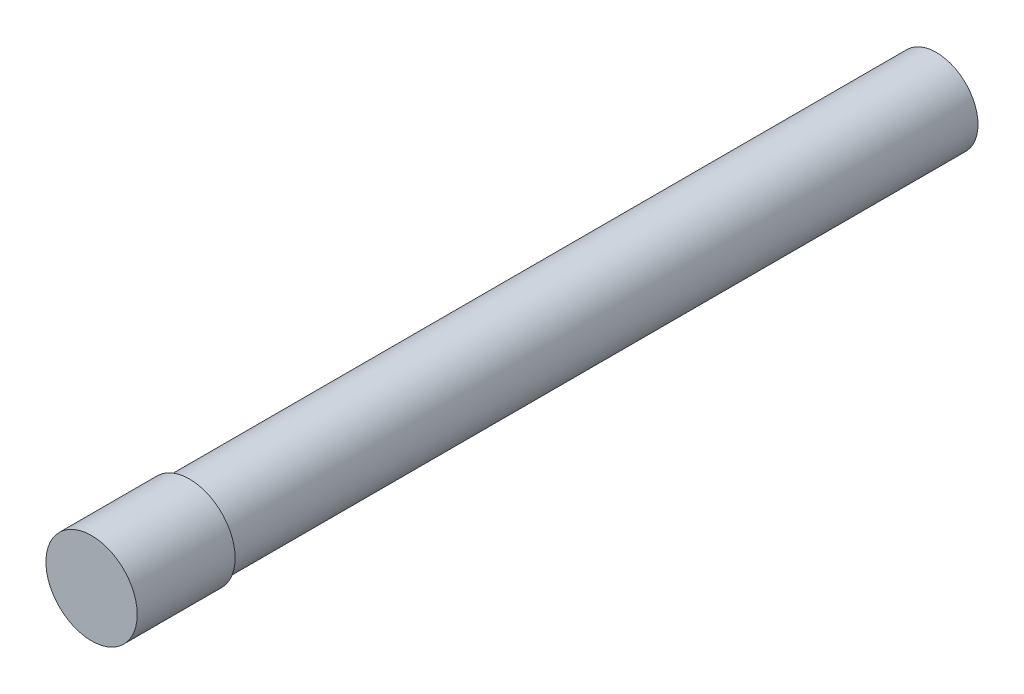
from build123d import *

# Parameters (mm, degrees)
SKETCH1_R           = 25.081999049
BOSS_EXTRUDE1_DEPTH = 450
SKETCH2_R           = 27.5
BOSS_EXTRUDE2_DEPTH = 59


with BuildPart() as part:
    # Sketch1 → Boss-Extrude1 (new body)
    with BuildSketch(Plane.XY):
        Circle(SKETCH1_R)
    extrude(amount=-BOSS_EXTRUDE1_DEPTH)

    # Sketch2 → Boss-Extrude2 (add)
    with BuildSketch(Plane.XY):
        Circle(SKETCH2_R)
    extrude(amount=BOSS_EXTRUDE2_DEPTH)


solid = part.part
